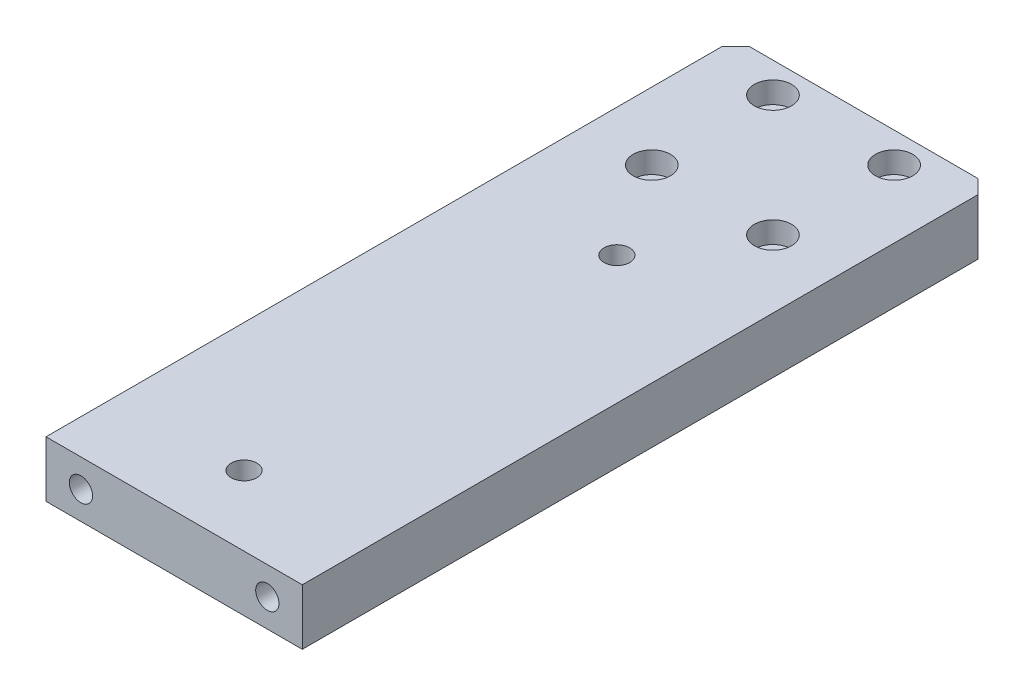
from build123d import *

# Parameters (mm, degrees)
SKETCH_1_W                = 55
SKETCH_1_H                = 148
EXTRUDE_1_DEPTH           = 6
CHAMFER_1_SIZE            = 3
HOLE_WIZARD_1_D           = 4.5
HOLE_WIZARD_1_CBORE_D     = 8
HOLE_WIZARD_1_CBORE_DEPTH = 4.6
HOLE_WIZARD_M6_1_D        = 5
HOLE_WIZARD_M6_1_DEPTH    = 15
HOLE_WIZARD_M6_1_TIP      = 1.502151548
HOLE_WIZARD_2_D           = 5.5
HOLE_WIZARD_2_CBORE_D     = 10
HOLE_WIZARD_2_CBORE_DEPTH = 5.7


with BuildPart() as part:
    # 草图1 → 凸台-拉伸1 (new, symmetric)
    with BuildSketch(Plane(origin=(0, 0, 0), x_dir=(1, 0, 0), z_dir=(0, 1, 0))):
        Rectangle(SKETCH_1_W, SKETCH_1_H)
    extrude(amount=EXTRUDE_1_DEPTH, both=True)

    # 倒角1
    chamfer_1_edges = [part.edges().sort_by_distance(p)[0] for p in [
        (-27.5, 0, -74),
        (27.5, 0, -74),
    ]]
    chamfer(chamfer_1_edges, length=CHAMFER_1_SIZE)

    # 打孔尺寸(%根据)内六角圆柱头螺钉的类型1 (through all)
    with Locations(Plane(origin=(0, 6, 0), x_dir=(1, 0, 0), z_dir=(0, 1, 0))):
        with Locations((13, 41.5), (13, 67.5), (-13, 67.5), (-13, 41.5)):
            CounterBoreHole(HOLE_WIZARD_1_D / 2, HOLE_WIZARD_1_CBORE_D / 2, HOLE_WIZARD_1_CBORE_DEPTH)

    # M6 螺纹孔1
    with Locations(Plane.XY.offset(74)):
        with Locations((20, 0), (-20, 0)):
            Hole(HOLE_WIZARD_M6_1_D / 2, depth=HOLE_WIZARD_M6_1_DEPTH)
            with Locations((0, 0, -(HOLE_WIZARD_M6_1_DEPTH + HOLE_WIZARD_M6_1_TIP / 2))):  # 118° drill point
                Cone(0, HOLE_WIZARD_M6_1_D / 2, HOLE_WIZARD_M6_1_TIP, mode=Mode.SUBTRACT)

    # 打孔尺寸(%根据)内六角圆柱头螺钉的类型2 (through all)
    with Locations(Plane.XZ.offset(6)):
        with Locations((0, 59), (0, -21)):
            CounterBoreHole(HOLE_WIZARD_2_D / 2, HOLE_WIZARD_2_CBORE_D / 2, HOLE_WIZARD_2_CBORE_DEPTH)


solid = part.part
